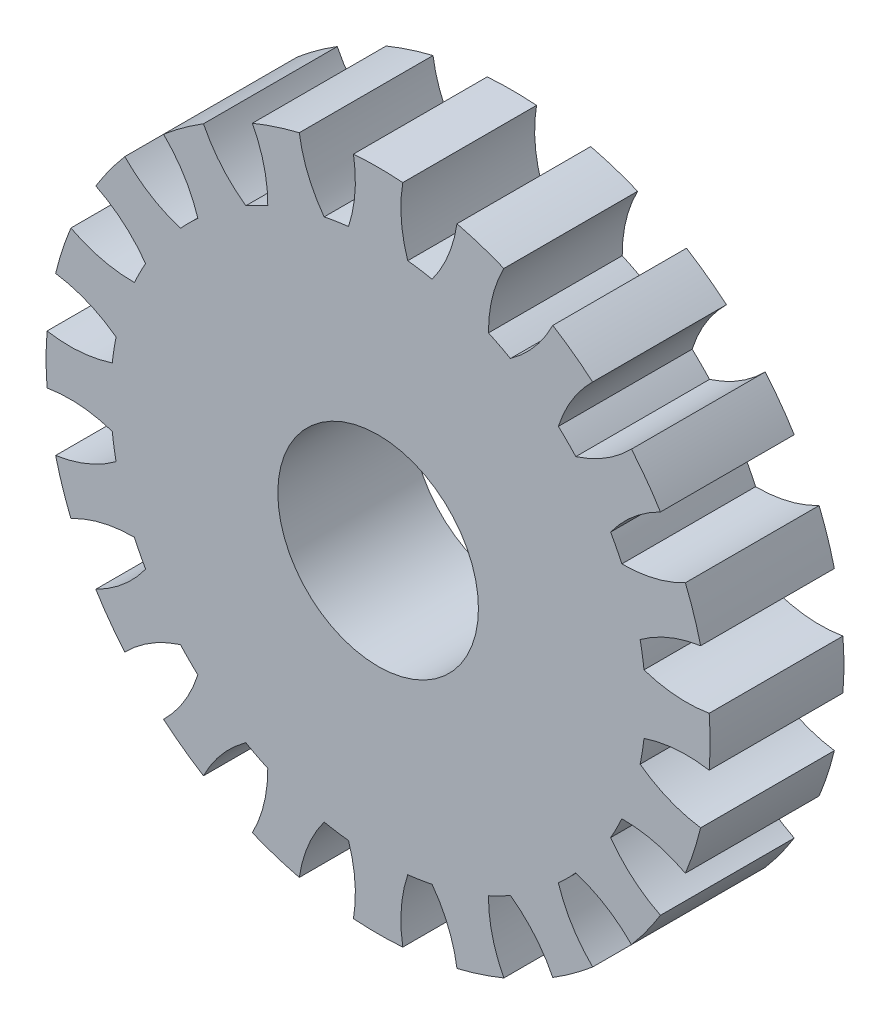
from build123d import *

# Parameters (mm, degrees)
SKETCH1_R           = 40
BOSS_EXTRUDE1_DEPTH = 10
CUT_EXTRUDE1_REACH  = 62
SKETCH2_R           = 15
BOSS_EXTRUDE2_DEPTH = 10
CIRPATTERN1_COUNT   = 20
SKETCH5_OUTSIDE_W   = 133.242
SKETCH5_OUTSIDE_H   = 133.242
SKETCH5_OUTSIDE_R   = 49.640577174
CUT_EXTRUDE4_DEPTH  = 53


with BuildPart() as part:
    # Sketch1 → Boss-Extrude1 (new, symmetric)
    with BuildSketch(Plane.XY):
        Circle(SKETCH1_R)
    extrude(amount=BOSS_EXTRUDE1_DEPTH, both=True)

    # Sketch2 → Cut-Extrude1 (cut, up to next)
    with BuildSketch(Plane.XY.offset(10), mode=Mode.PRIVATE) as cut_extrude1_sk1:
        Circle(SKETCH2_R)
    cut_extrude1_tool1 = extrude(cut_extrude1_sk1.sketch, amount=-CUT_EXTRUDE1_REACH, mode=Mode.PRIVATE) & part.part
    add(cut_extrude1_tool1.solids().sort_by_distance((0, 0, 10))[0], mode=Mode.SUBTRACT)

    # Sketch4 → Boss-Extrude2 (add, symmetric)
    with BuildSketch(Plane.XY):
        with BuildLine():
            ThreePointArc((3.963482067, 50.835965639), (3.418931143, 45.262287362), (4.429441361, 39.753994129))
            ThreePointArc((4.429441361, 39.753994129), (0, 40), (-4.429441361, 39.753994129))
            ThreePointArc((-4.429441361, 39.753994129), (-3.418931143, 45.262287362), (-3.963482067, 50.835965639))
            ThreePointArc((-3.963482067, 50.835965639), (0, 51.045354515), (3.963482067, 50.835965639))
        make_face()
    boss_extrude2 = extrude(amount=BOSS_EXTRUDE2_DEPTH, both=True)

    # CirPattern1: Boss-Extrude2 ×20 about axis
    cirpattern1_axis = Axis((0, 0, 0), (0, 0, 1))
    for i in range(1, CIRPATTERN1_COUNT):
        add(boss_extrude2.rotate(cirpattern1_axis, i * 360 / CIRPATTERN1_COUNT))

    # Sketch5 outside → Cut-Extrude4 (cut)
    with BuildSketch(Plane(origin=(0, 0, -10), x_dir=(-1, 0, 0), z_dir=(0, 0, -1))):
        Rectangle(SKETCH5_OUTSIDE_W, SKETCH5_OUTSIDE_H)
        Circle(SKETCH5_OUTSIDE_R, mode=Mode.SUBTRACT)
    extrude(amount=-CUT_EXTRUDE4_DEPTH, mode=Mode.SUBTRACT)


solid = part.part
